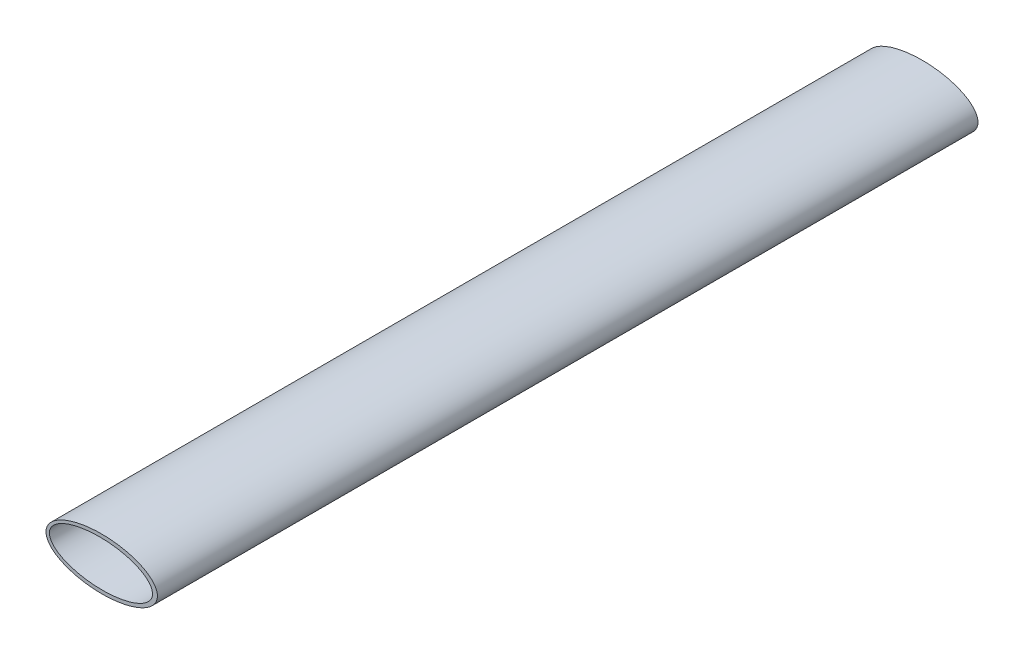
from build123d import *

# Parameters (mm, degrees)
SKETCH1_RX          = 23.625
SKETCH1_RY          = 11
SKETCH1_RX_2        = 21.86795069
SKETCH1_RY_2        = 9.506412044
BOSS_EXTRUDE1_DEPTH = 348


with BuildPart() as part:
    # Sketch1 → Boss-Extrude1 (new body)
    with BuildSketch(Plane(origin=(0, 0, 55.201283758), x_dir=(-1, 0, 0), z_dir=(0, 0, -1))):
        with Locations(Location((539, 967.2), (0, 0, 180))):
            Ellipse(SKETCH1_RX, SKETCH1_RY)
        with Locations(Location((539.318959601, 967.197494981), (0, 0, -179.186603951))):
            Ellipse(SKETCH1_RX_2, SKETCH1_RY_2, mode=Mode.SUBTRACT)
    extrude(amount=-BOSS_EXTRUDE1_DEPTH)


solid = part.part
